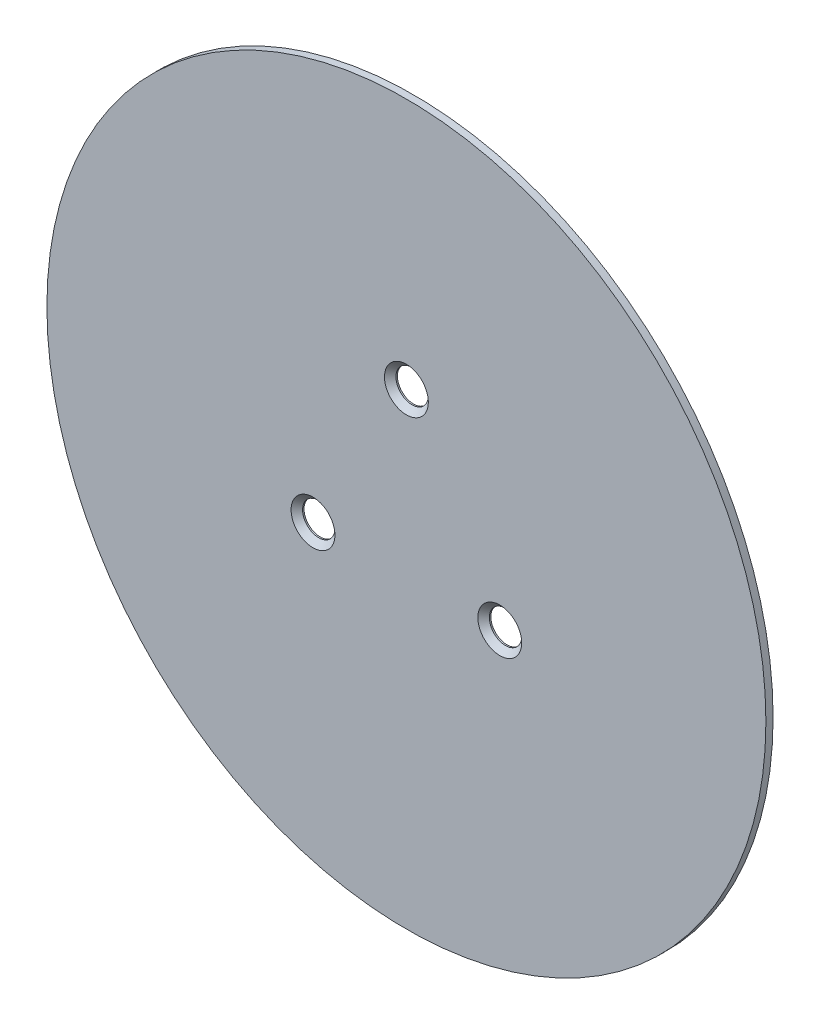
from build123d import *

# Parameters (mm, degrees)
SKETCH_1_R      = 50
SKETCH_1_R_2    = 2.25
EXTRUDE_1_DEPTH = 1
CHAMFER_1_SIZE  = 0.8


with BuildPart() as part:
    # 草图1 → 凸台-拉伸1 (new body)
    with BuildSketch(Plane.XY):
        Circle(SKETCH_1_R)
        with Locations((0, 15)):
            Circle(SKETCH_1_R_2, mode=Mode.SUBTRACT)
        with Locations((12.990381057, -7.5)):
            Circle(SKETCH_1_R_2, mode=Mode.SUBTRACT)
        with Locations((-12.990381057, -7.5)):
            Circle(SKETCH_1_R_2, mode=Mode.SUBTRACT)
    extrude(amount=EXTRUDE_1_DEPTH)

    # 倒角1
    chamfer_1_edges = [part.edges().sort_by_distance(p)[0] for p in [
        (-15.240381057, -7.5, 1),
        (-2.25, 15, 1),
        (10.740381057, -7.5, 1),
    ]]
    chamfer(chamfer_1_edges, length=CHAMFER_1_SIZE)


solid = part.part
